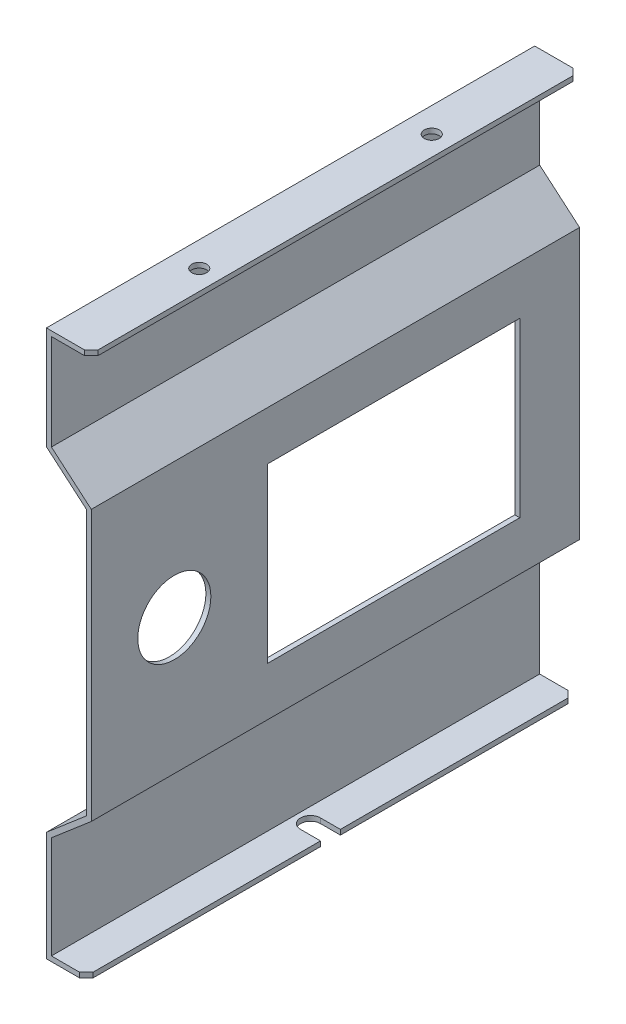
from build123d import *

# Parameters (mm, degrees)
EXTRUDE_THIN1_DEPTH = 73.5
SKETCH2_W           = 76
SKETCH2_H           = 52
CUT_EXTRUDE1_DEPTH  = 10
CHAMFER1_SIZE       = 2
CUT_EXTRUDE3_DEPTH  = 5
SKETCH7_R           = 11
CUT_EXTRUDE4_DEPTH  = 10
SKETCH8_R           = 2.25
CUT_EXTRUDE5_DEPTH  = 10


with BuildPart() as part:
    # Sketch1 → Extrude-Thin1 (new, symmetric)
    with BuildSketch(Plane.XY):
        Polygon((12, 0), (0, 0), (0, 33), (12, 43.248968226), (12, 123.248968226), (0, 133.497936451), (0, 164.497936451), (13.5, 164.497936451), (13.5, 162.997936451), (1.5, 162.997936451), (1.5, 134.189445923), (13.5, 123.940477697), (13.5, 42.557458754), (1.5, 32.308490528), (1.5, 1.5), (12, 1.5), align=None)
    extrude(amount=EXTRUDE_THIN1_DEPTH, both=True)

    # Sketch2 → Cut-Extrude1 (cut)
    with BuildSketch(Plane.ZY.offset(-12)):
        with Locations((-17.5, 83.248968226)):
            Rectangle(SKETCH2_W, SKETCH2_H)
    extrude(amount=-CUT_EXTRUDE1_DEPTH, mode=Mode.SUBTRACT)

    # Chamfer1
    chamfer1_edges = [part.edges().sort_by_distance(p)[0] for p in [
        (13.5, 163.747936451, -73.5),
        (12, 0.75, -73.5),
        (13.5, 163.747936451, 73.5),
        (12, 0.75, 73.5),
    ]]
    chamfer(chamfer1_edges, length=CHAMFER1_SIZE)

    # Sketch6 → Cut-Extrude3 (cut)
    with BuildSketch(Plane.XZ):
        with BuildLine():
            Line((6, 3), (12, 3))
            ThreePointArc((12, 3), (15, 0), (12, -3))
            Line((12, -3), (6, -3))
            ThreePointArc((6, -3), (3, 0), (6, 3))
        make_face()
    extrude(amount=-CUT_EXTRUDE3_DEPTH, mode=Mode.SUBTRACT)

    # Sketch7 → Cut-Extrude4 (cut)
    with BuildSketch(Plane.ZY.offset(-12)):
        with Locations(Location((48.5, 83.248968226, 0), (0, 0, 270))):
            Circle(SKETCH7_R)
    extrude(amount=-CUT_EXTRUDE4_DEPTH, mode=Mode.SUBTRACT)

    # Sketch8 → Cut-Extrude5 (cut)
    with BuildSketch(Plane(origin=(0, 164.497936451, 0), x_dir=(1, 0, 0), z_dir=(0, 1, 0))):
        with Locations(Location((7.5, 35, 0), (0, 0, 180))):
            Circle(SKETCH8_R)
    cut_extrude5 = extrude(amount=-CUT_EXTRUDE5_DEPTH, mode=Mode.SUBTRACT)

    # Mirror1: Cut-Extrude5 across plane
    add(cut_extrude5.mirror(Plane.XY), mode=Mode.SUBTRACT)


solid = part.part
